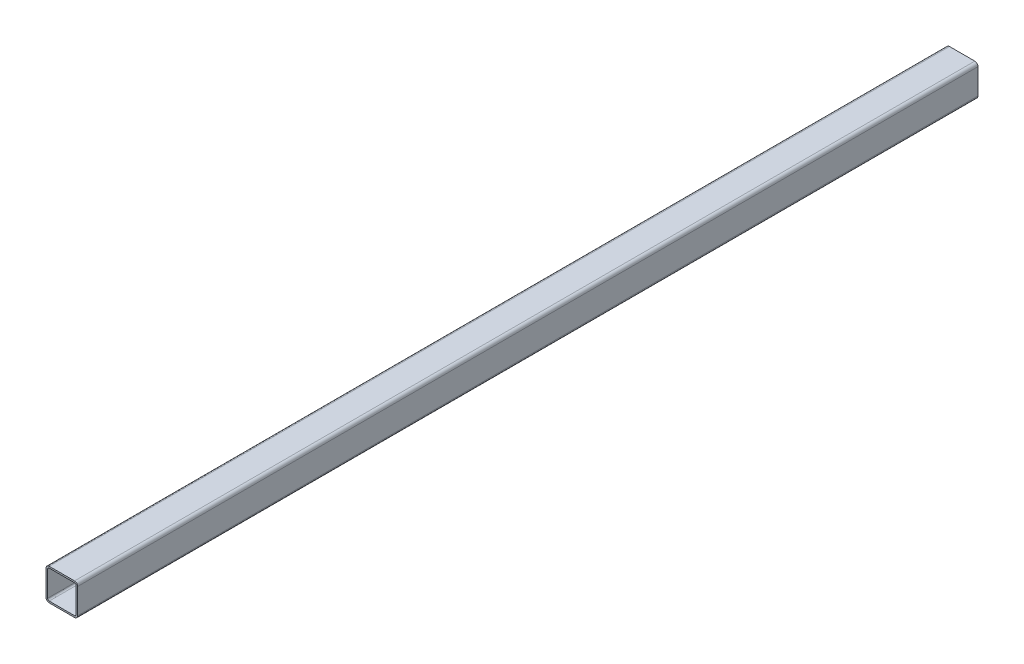
from build123d import *

# Parameters (mm, degrees)
BOSS_EXTRUDE1_DEPTH = 2840


with BuildPart() as part:
    # Sketch1 → Boss-Extrude1 (new body)
    with BuildSketch(Plane.XY):
        with BuildLine():
            Line((10, 0), (90, 0))
            ThreePointArc((90, 0), (97.071067812, 2.928932188), (100, 10))
            Line((100, 10), (100, 90))
            ThreePointArc((100, 90), (97.071067812, 97.071067812), (90, 100))
            Line((90, 100), (10, 100))
            ThreePointArc((10, 100), (2.928932188, 97.071067812), (0, 90))
            Line((0, 90), (0, 10))
            ThreePointArc((0, 10), (2.928932188, 2.928932188), (10, 0))
        make_face()
        with BuildLine():
            Line((10, 95), (90, 95))
            ThreePointArc((90, 95), (93.535533906, 93.535533906), (95, 90))
            Line((95, 90), (95, 10))
            ThreePointArc((95, 10), (93.535533906, 6.464466094), (90, 5))
            Line((90, 5), (10, 5))
            ThreePointArc((10, 5), (6.464466094, 6.464466094), (5, 10))
            Line((5, 10), (5, 90))
            ThreePointArc((5, 90), (6.464466094, 93.535533906), (10, 95))
        make_face(mode=Mode.SUBTRACT)
    extrude(amount=BOSS_EXTRUDE1_DEPTH)


solid = part.part
